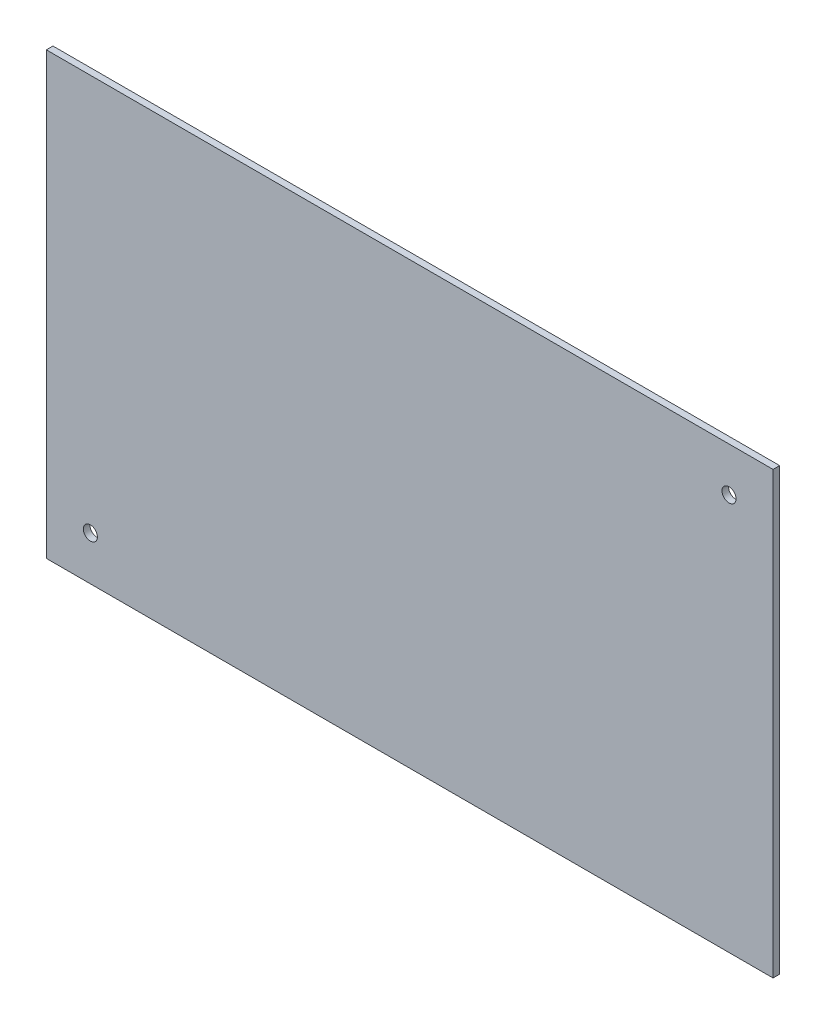
SolidWorks part; units mm, degrees
ref_plane "前视基准面" through (0, 0, 0) normal (0, 0, 1) x (1, 0, 0)
ref_plane "上视基准面" through (0, 0, 0) normal (0, 1, 0) x (1, 0, 0)
ref_plane "右视基准面" through (0, 0, 0) normal (1, 0, 0) x (0, 0, -1)
other "Configuration Table"
sketch "草图1" plane through (0, 0, 0) normal (0, 0, 1) x (1, 0, 0)
  line L0 (-165, -100) -> (165, -100)
  line L1 (165, -100) -> (165, 100)
  line L2 (165, 100) -> (-165, 100)
  line L3 (-165, 100) -> (-165, -100)
  point P0 (0, 0)
  dimension "D1" = 165
  dimension "D2" = 330
  dimension "D3" = 100
  dimension "D4" = 200
extrude "凸台-拉伸1" add sketch "草图1" against normal mid plane 3
sketch "草图2" plane through (0, 0, 0) normal (0, 0, 1) x (1, 0, 0)
  circle A0 centre (-145, -80) radius 3.2
  circle A1 centre (145, 80) radius 3.2
  point P0 (0, 0)
  dimension "D1" = 6.4
  dimension "D2" = 6.4
  dimension "D3" = 145
  dimension "D4" = 290
  dimension "D5" = 80
  dimension "D6" = 160
extrude "切除-拉伸1" cut sketch "草图2" against normal mid plane 23
